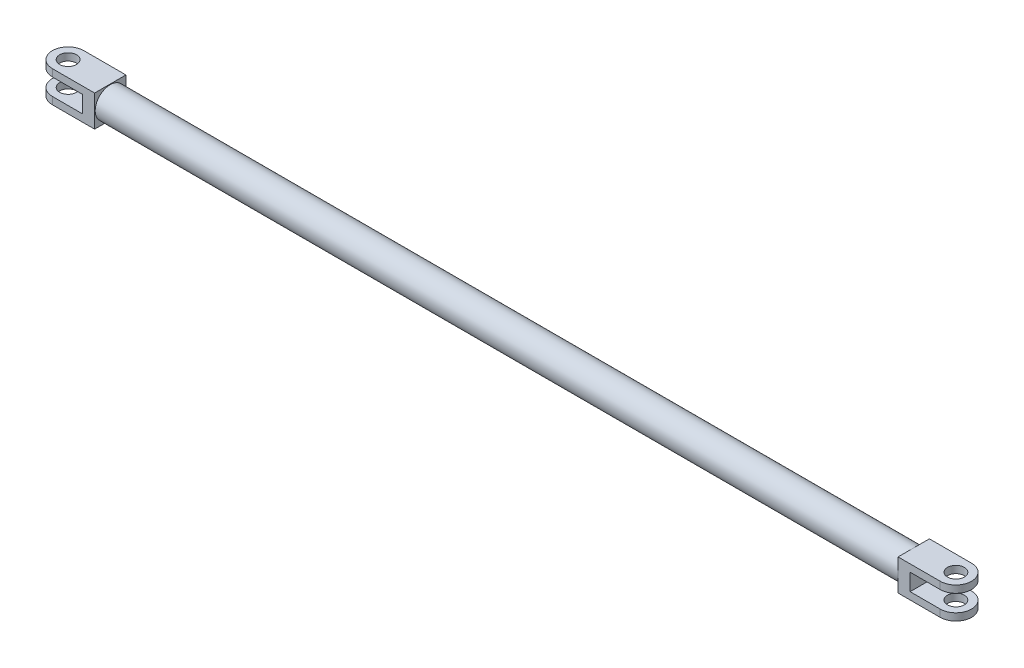
from build123d import *

# Parameters (mm, degrees)
SKETCH_1_R               = 7
EXTRUDE_1_DEPTH          = 13
CUT_EXTRUDE_1_DEPTH      = 40.534794802
CUT_EXTRUDE_1_DEPTH_BACK = 40.534794802
SKETCH_2_W               = 50
SKETCH_2_H               = 14
SKETCH_3_R               = 12.5
SKETCH_3_R_2             = 9.5
EXTRUDE_2_DEPTH          = 667


with BuildPart() as part:
    # 草图1 → 凸台-拉伸1 (new, symmetric)
    with BuildSketch(Plane(origin=(0, 0, 0), x_dir=(1, 0, 0), z_dir=(0, 1, 0))):
        with BuildLine():
            Line((0, 13), (35, 13))
            Line((35, 13), (35, -13))
            Line((35, -13), (0, -13))
            ThreePointArc((0, -13), (-13, 0), (0, 13))
        make_face()
        with Locations(Location((0, 0, 0), (0, 0, 90))):
            Circle(SKETCH_1_R, mode=Mode.SUBTRACT)
    extrude(amount=EXTRUDE_1_DEPTH, both=True)

    # 草图2 → 切除-拉伸1 (cut, two sides: drawn at the far end of the back side and taken through both)
    with BuildSketch(Plane.XY.offset(-CUT_EXTRUDE_1_DEPTH_BACK)):
        Rectangle(SKETCH_2_W, SKETCH_2_H)
    extrude(amount=CUT_EXTRUDE_1_DEPTH + CUT_EXTRUDE_1_DEPTH_BACK, mode=Mode.SUBTRACT)


with BuildPart() as body_2:
    # 草图3 → 凸台-拉伸2 (new body)
    with BuildSketch(Plane(origin=(35, 0, 0), x_dir=(0, 0, -1), z_dir=(1, 0, 0))):
        Circle(SKETCH_3_R)
        Circle(SKETCH_3_R_2, mode=Mode.SUBTRACT)
    extrude(amount=EXTRUDE_2_DEPTH)


with BuildPart() as body_3:
    # 镜向1: mirrored copy
    add(part.part.mirror(Plane(origin=(368.5, 0, 0), x_dir=(0, 0, 1), z_dir=(1, 0, 0))))


solid = Compound([part.part, body_2.part, body_3.part])
